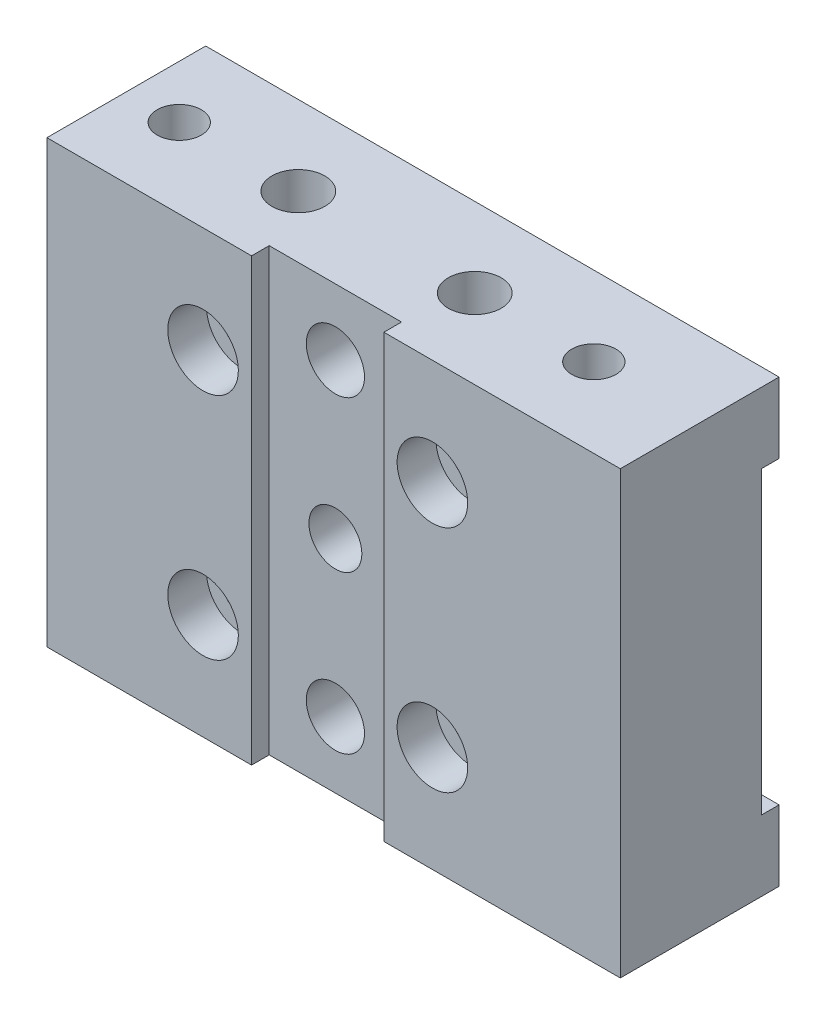
SolidWorks part; units mm, degrees
material "#45(1.1191)"
ref_plane "前视基准面" through (0, 0, 0) normal (0, 0, 1) x (1, 0, 0)
ref_plane "上视基准面" through (0, 0, 0) normal (0, 1, 0) x (1, 0, 0)
ref_plane "右视基准面" through (0, 0, 0) normal (1, 0, 0) x (0, 0, -1)
sketch "草图1" plane through (0, 0, 0) normal (0, 0, 1) x (1, 0, 0)
  line L1 (-32.5, 25) -> (32.5, 25)
  line L2 (-32.5, 25) -> (-32.5, -25)
  line L3 (-32.5, -25) -> (32.5, -25)
  line L4 (32.5, 25) -> (32.5, -25)
  line L5 (-32.5, 25) -> (32.5, -25) construction
  line L6 (-32.5, -25) -> (32.5, 25) construction
  point P0 (0, 0)
  dimension "D1" = 50
  dimension "D2" = 65
extrude "凸台-拉伸1" add sketch "草图1" along normal mid plane 18
sketch "草图2" plane through (0, 0, 9) normal (0, 0, 1) x (1, 0, 0)
  line L0 (32.5, 0) -> (-32.5, 0) construction
  line L1 (32.5, -25) -> (32.5, 25) construction
  line L2 (-32.5, 25) -> (-32.5, -25) construction
  point P0 (28.5, 0)
  point P2 (-7.5, 0)
  point P4 (-43.5, 0)
  dimension "D1" = 4
  dimension "D2" = 36
  dimension "D3" = 36
hole_wizard "M4 间隙孔1" positions "草图2" profile "草图3" hole size "M4" standard "GB"
sketch "草图3" plane through (33.5, 0, 7.5) normal (1, 0, 0) x (0, -1, 0)
  line L0 (0, 0) -> (0, 15)
  line L1 (0, 15) -> (2.25, 15)
  line L2 (2.25, 15) -> (2.25, 0)
  line L5 (2.25, 0) -> (0, 0)
  line L11 (0, -6.35) -> (0, 107.95) construction
  dimension "通孔孔直径" = 4.5
  dimension "通孔孔深度" = 15
sketch "草图4" plane through (32.5, 0, 0) normal (1, 0, 0) x (0, 0, -1)
  line L1 (7, 17) -> (9, 17)
  line L2 (7, 17) -> (7, -17)
  line L3 (7, -17) -> (9, -17)
  line L4 (9, 17) -> (9, -17)
  line L5 (7, 17) -> (9, -17) construction
  line L6 (7, -17) -> (9, 17) construction
  line L7 (9, -25) -> (9, 25) construction
  point P0 (8, 0)
  dimension "D1" = 34
  dimension "D2" = 2
extrude "切除-拉伸1" cut sketch "草图4" against normal through all
sketch "草图5" plane through (0, 0, 9) normal (0, 0, 1) x (1, 0, 0)
  line L0 (32.5, -7.25) -> (27.5, -7.25)
  line L1 (32.5, -25) -> (32.5, 25) construction
  line L2 (27.5, -7.25) -> (27.5, -9.75)
  line L3 (27.5, -9.75) -> (19, -9.75)
  line L4 (19, -9.75) -> (19, 9.75)
  line L5 (0, 0) -> (32.5, 0) construction
  line L6 (32.5, -7.25) -> (32.5, 7.25)
  line L7 (27.5, 9.75) -> (19, 9.75)
  line L8 (27.5, 7.25) -> (27.5, 9.75)
  line L9 (32.5, 7.25) -> (27.5, 7.25)
  point P13 (16.25, 0)
  dimension "D1" = 14.5
  dimension "D2" = 19.5
  dimension "D3" = 5
  dimension "D4" = 8.5
extrude "切除-拉伸2" [suppressed] cut sketch "草图5" against normal through all
sketch "草图6" plane through (0, 0, 9) normal (0, 0, 1) x (1, 0, 0)
  point P0 (11.2, -13)
  point P3 (-14.8, -13)
  point P6 (-14.8, 13)
  point P9 (11.2, 13)
hole_wizard "M4 六角凹头螺钉的柱形沉头孔1" positions "草图6" profile "草图7" counterbore size "M4" standard "ISO" end condition through all
sketch "草图7" plane through (11.2, -13, 9) normal (1, 0, 0) x (0, -1, 0)
  line L0 (0, 0) -> (0, 18)
  line L1 (0, 18) -> (2.25, 18)
  line L3 (2.25, 18) -> (2.25, 4.4)
  line L4 (2.25, 4.4) -> (4, 4.4)
  line L5 (4, 4.4) -> (4, 0)
  line L7 (4, 0) -> (0, 0)
  line L11 (0, -6.35) -> (0, 107.95) construction
  dimension "通孔孔直径" = 4.5
  dimension "通孔孔深度" = 18
  dimension "柱形沉头孔直径" = 8
  dimension "柱形沉头孔深度" = 4.4
sketch "草图8" plane through (0, 0, 9) normal (0, 0, 1) x (1, 0, 0)
  line L0 (-32.5, -25) -> (32.5, -25) construction
  line L1 (-9.3, 25) -> (5.7, 25)
  line L2 (-9.3, 25) -> (-9.3, -25)
  line L3 (-9.3, -25) -> (5.7, -25)
  line L4 (5.7, 25) -> (5.7, -25)
  line L5 (-9.3, 25) -> (5.7, -25) construction
  line L6 (-9.3, -25) -> (5.7, 25) construction
  line L7 (-32.5, 25) -> (-32.5, -25) construction
  line L8 (32.5, 25) -> (-32.5, 25) construction
  point P0 (-1.8, 0)
  dimension "D1" = 15
  dimension "D2" = 30.7
extrude "切除-拉伸3" cut sketch "草图8" against normal blind 2
sketch "草图9" plane through (0, 0, 7) normal (0, 0, 1) x (1, 0, 0)
  line L0 (-9.3, 0) -> (5.7, 0) construction
  line L1 (-9.3, 25) -> (-9.3, -25) construction
  line L2 (5.7, -25) -> (5.7, 25) construction
  point P0 (-1.8, 0)
hole_wizard "Ø6.0mm 暗销孔1" positions "草图9" profile "草图10" hole size "Ø6.0" standard "ISO"
sketch "草图10" plane through (-1.8, 0, 7) normal (1, 0, 0) x (0, -1, 0)
  line L0 (0, 0) -> (0, 8.8026)
  line L1 (0, 8.8026) -> (3, 7)
  line L2 (3, 7) -> (3, 0)
  line L5 (3, 0) -> (0, 0)
  line L10 (0, 8.8026) -> (-3, 7) construction
  line L11 (0, -6.35) -> (0, 107.95) construction
  dimension "孔直径" = 6
  dimension "孔深度" = 7
  dimension "导头角度" = 118
hole_wizard "M6 六角凹头螺钉的柱形沉头孔2" positions "草图13" profile "草图14" counterbore size "M6" standard "ISO" end condition through all
sketch "草图13" plane through (0, 0, -9) normal (0, 0, -1) x (-1, 0, 0)
  point P0 (1.8, 17.5)
  point P3 (1.8, -17.5)
sketch "草图14" plane through (-1.8, 17.5, -9) normal (1, 0, 0) x (0, 1, 0)
  line L0 (0, 0) -> (0, 18)
  line L1 (0, 18) -> (3.3, 18)
  line L3 (3.3, 18) -> (3.3, 9)
  line L4 (3.3, 9) -> (5.5, 9)
  line L5 (5.5, 9) -> (5.5, 0)
  line L7 (5.5, 0) -> (0, 0)
  line L11 (0, -6.35) -> (0, 107.95) construction
  dimension "通孔孔直径" = 6.6
  dimension "通孔孔深度" = 18
  dimension "柱形沉头孔直径" = 11
  dimension "柱形沉头孔深度" = 9
sketch "草图15" plane through (0, 25, 0) normal (0, 1, 0) x (1, 0, 0)
  point P0 (20.5, 0)
  point P3 (-26.5, 0)
hole_wizard "M6 螺纹孔1" positions "草图15" profile "草图16" tap size "M6" standard "ISO"
sketch "草图16" plane through (20.5, 25, 0) normal (1, 0, 0) x (0, 0, 1)
  line L0 (0, 0) -> (0, 16.5022)
  line L1 (0, 16.5022) -> (2.5, 15)
  line L2 (2.5, 15) -> (2.5, 0)
  line L5 (2.5, 0) -> (0, 0)
  line L10 (0, 16.5022) -> (-2.5, 15) construction
  line L11 (0, -6.35) -> (0, 107.95) construction
  dimension "螺纹孔钻头直径" = 5
  dimension "螺纹孔钻头深度" = 15
  dimension "导头角度" = 118
cosmetic thread "孔螺蚊线1" parameters "D1"=12, "D2"=6
cosmetic thread "孔螺蚊线2" parameters "D1"=12, "D2"=6
sketch "草图17" plane through (0, 25, 0) normal (0, 1, 0) x (1, 0, 0)
  point P0 (7, 0)
  point P3 (-13, 0)
hole_wizard "Ø6.0mm 暗销孔2" positions "草图17" profile "草图18" hole size "Ø6.0" standard "ISO"
sketch "草图18" plane through (7, 25, 0) normal (1, 0, 0) x (0, 0, 1)
  line L0 (0, 0) -> (0, 7.8026)
  line L1 (0, 7.8026) -> (3, 6)
  line L2 (3, 6) -> (3, 0)
  line L5 (3, 0) -> (0, 0)
  line L10 (0, 7.8026) -> (-3, 6) construction
  line L11 (0, -6.35) -> (0, 107.95) construction
  dimension "孔直径" = 6
  dimension "孔深度" = 6
  dimension "导头角度" = 118
